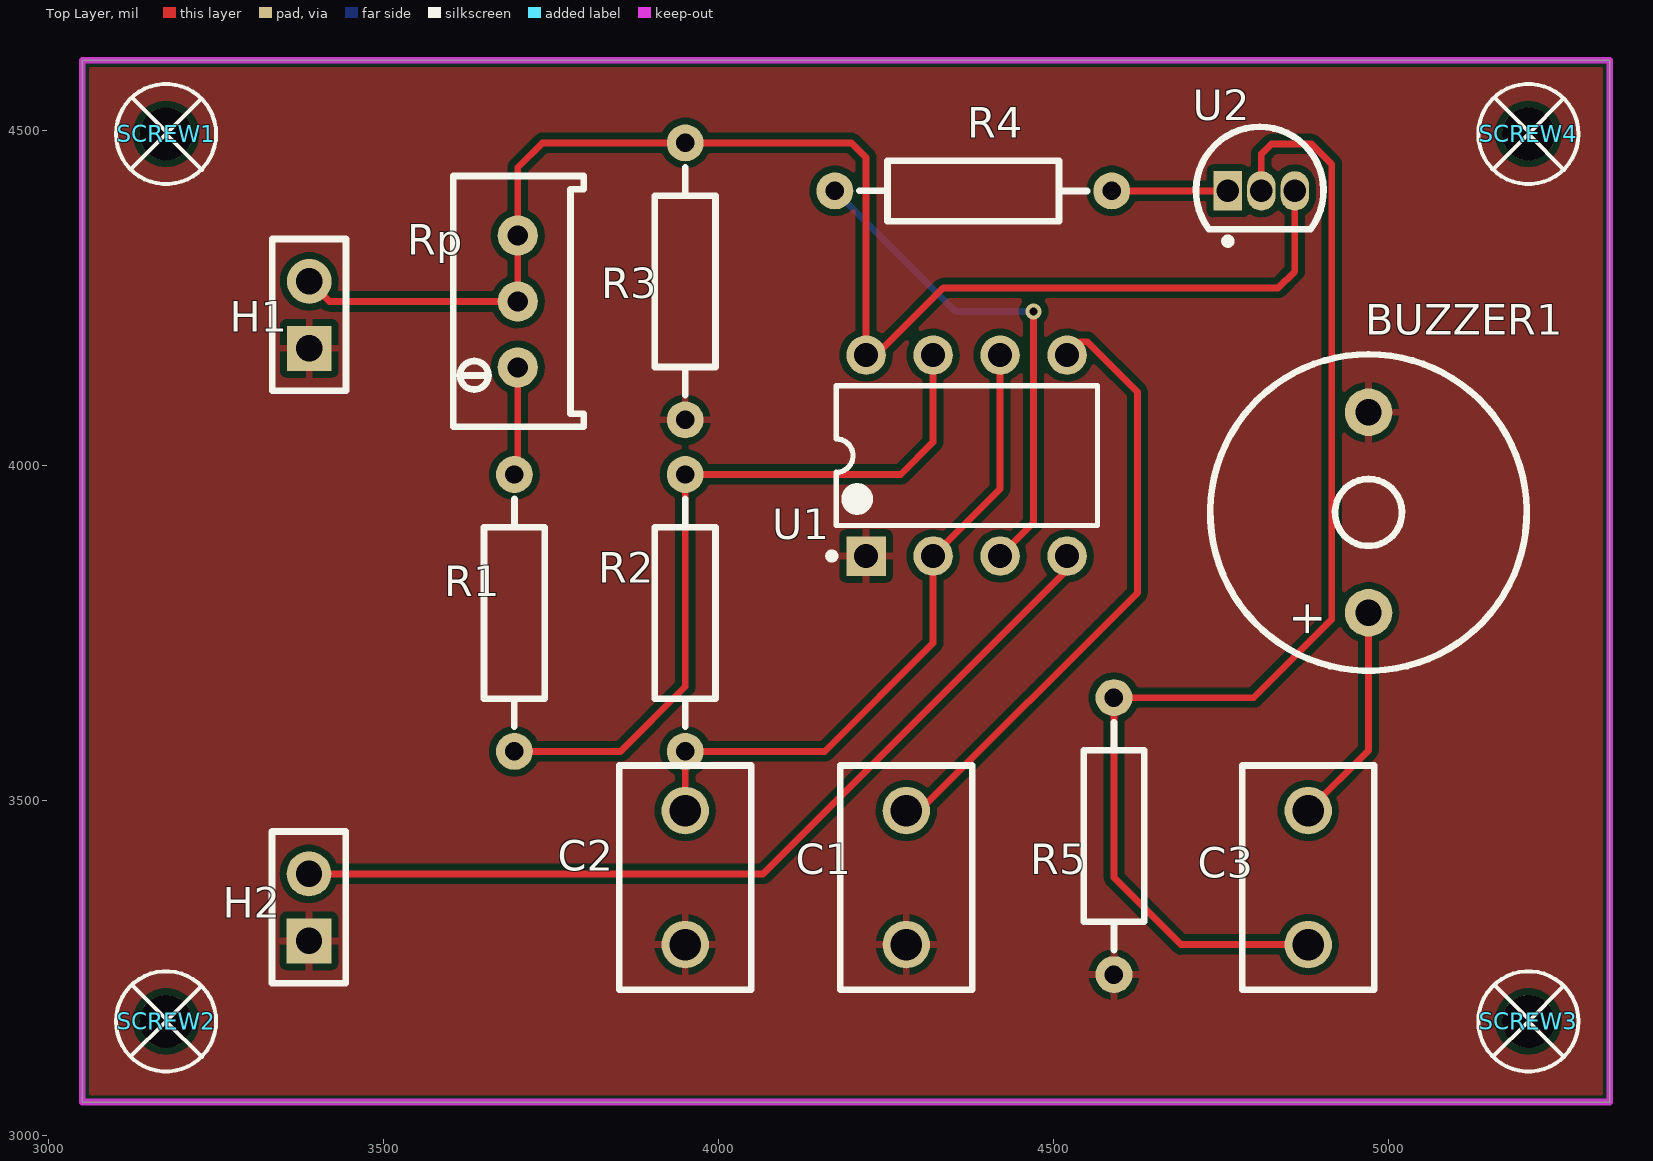
[diagram p0: Top Layer view]
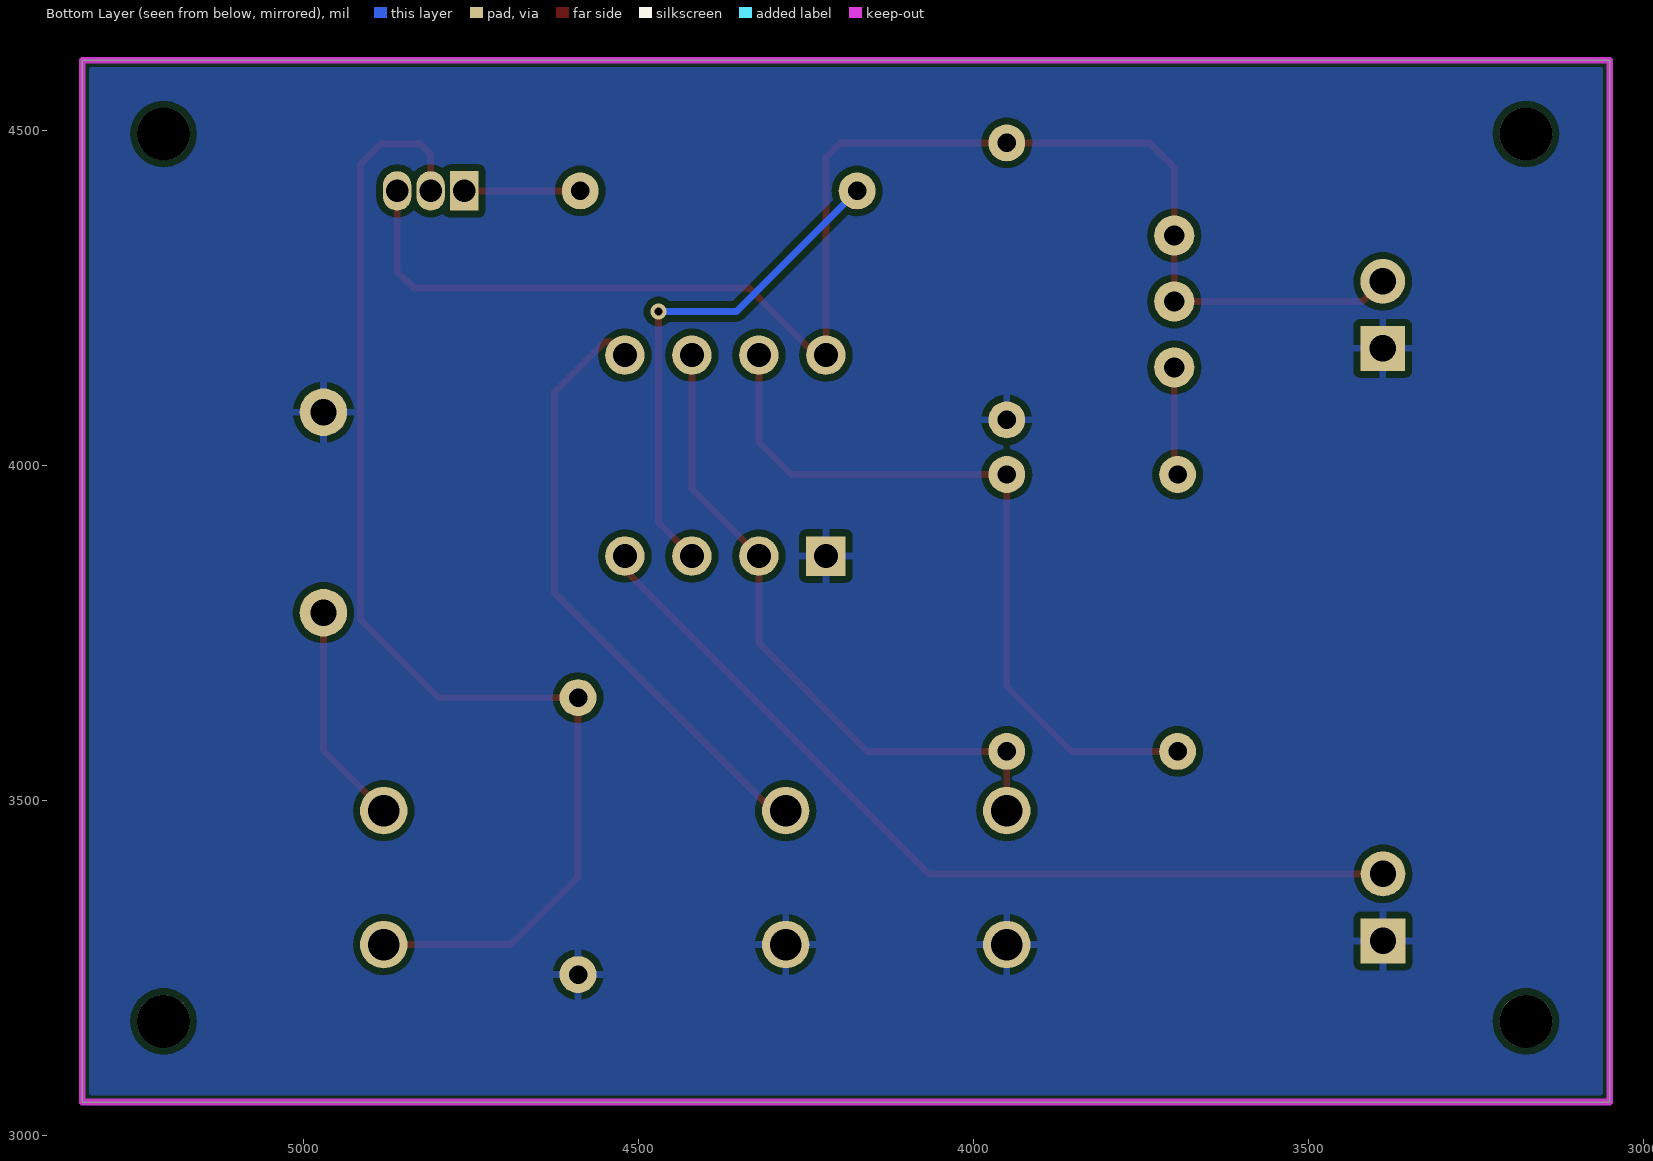
[diagram p1: Bottom Layer view, seen from below]
# Altium PCB MISC51754.pcbdoc
Units mil, origin at the board's own origin, x right, y up, seen from the top; angles counter-clockwise.
Board outline 2280 x 1555 mil, 2 copper layers (Top Layer, Bottom Layer), stack 62.206 mil thick; 18 components, 11 nets, 40 pads, 1 vias.

## Layer stack, top to bottom
Top Solder Mask Layer: solder mask 0.394, Dk 3.3
Top Layer: signal copper 1.379
Dielectric1: surface 59.449, FR4, Dk 4.5
Bottom Layer: signal copper 1.378
Bottom Solder Mask Layer: solder mask 0.394, Dk 3.3

## Board outline
3050,4605 3050,3050 5330,3050 5330,4605

## Design rules (kind name [scope] priority, off if disabled: settings)
BoardOutlineClearance copperThickness2oz_1 [All] p2 off: genericclearance=7.99 ignorepadtopadclearanceinfootprint=FALSE except(0: Arc-SplitContinuation Track-SplitContinuation SMDPad-SplitContinuation THPad-SplitContinuation Via-SplitContinuation Fill-SplitContinuation Region-SplitContinuation Poly-SplitContinuation Text-SplitContinuation Hole-SplitContinuation; 5.98: SMDPad-CutoutEdge THPad-CutoutEdge Via-CutoutEdge Fill-CutoutEdge Region-CutoutEdge Text-CutoutEdge Hole-CutoutEdge; 10: Poly-OutlineEdge Poly-CutoutEdge; 11.81: Arc-OutlineEdge Track-OutlineEdge SMDPad-OutlineEdge THPad-OutlineEdge Via-OutlineEdge Fill-OutlineEdge Region-OutlineEdge Text-OutlineEdge Hole-OutlineEdge Arc-CutoutEdge Track-CutoutEdge)
BoardOutlineClearance Plane_innerPlane_1 [All] p4 off: genericclearance=4.02 ignorepadtopadclearanceinfootprint=FALSE except(0: Arc-SplitContinuation Track-SplitContinuation SMDPad-SplitContinuation THPad-SplitContinuation Via-SplitContinuation Fill-SplitContinuation Region-SplitContinuation Poly-SplitContinuation Text-SplitContinuation Hole-SplitContinuation; 5.98: SMDPad-CutoutEdge THPad-CutoutEdge Via-CutoutEdge Fill-CutoutEdge Region-CutoutEdge Text-CutoutEdge Hole-CutoutEdge; 10: Poly-OutlineEdge Poly-CutoutEdge; 11.81: Arc-OutlineEdge Track-OutlineEdge SMDPad-OutlineEdge THPad-OutlineEdge Via-OutlineEdge Fill-OutlineEdge Region-OutlineEdge Text-OutlineEdge Hole-OutlineEdge Arc-CutoutEdge Track-CutoutEdge)
BoardOutlineClearance Copper_copperRegion_1 [All] p6 off: genericclearance=4.02 ignorepadtopadclearanceinfootprint=FALSE except(0: Arc-SplitContinuation Track-SplitContinuation SMDPad-SplitContinuation THPad-SplitContinuation Via-SplitContinuation Fill-SplitContinuation Region-SplitContinuation Poly-SplitContinuation Text-SplitContinuation Hole-SplitContinuation; 5.98: SMDPad-CutoutEdge THPad-CutoutEdge Via-CutoutEdge Fill-CutoutEdge Region-CutoutEdge Text-CutoutEdge Hole-CutoutEdge; 10: Poly-OutlineEdge Poly-CutoutEdge; 11.81: Arc-OutlineEdge Track-OutlineEdge SMDPad-OutlineEdge THPad-OutlineEdge Via-OutlineEdge Fill-OutlineEdge Region-OutlineEdge Text-OutlineEdge Hole-OutlineEdge Arc-CutoutEdge Track-CutoutEdge)
BoardOutlineClearance copperThickness1oz_1 [All] p8: genericclearance=4.02 ignorepadtopadclearanceinfootprint=FALSE except(0: Arc-SplitContinuation Track-SplitContinuation SMDPad-SplitContinuation THPad-SplitContinuation Via-SplitContinuation Fill-SplitContinuation Region-SplitContinuation Poly-SplitContinuation Text-SplitContinuation Hole-SplitContinuation; 5.98: SMDPad-CutoutEdge THPad-CutoutEdge Via-CutoutEdge Fill-CutoutEdge Region-CutoutEdge Text-CutoutEdge Hole-CutoutEdge; 10: Poly-OutlineEdge Poly-CutoutEdge; 11.81: Arc-OutlineEdge Track-OutlineEdge SMDPad-OutlineEdge THPad-OutlineEdge Via-OutlineEdge Fill-OutlineEdge Region-OutlineEdge Text-OutlineEdge Hole-OutlineEdge Arc-CutoutEdge Track-CutoutEdge)
Clearance copperThickness2oz [All] p1 off: gap=7.99 ignorepadtopadclearanceinfootprint=FALSE except(5.98: SMDPad-Track SMDPad-SMDPad THPad-Track SMDPad-THPad THPad-THPad Track-Via SMDPad-Via THPad-Via Via-Via Fill-Track Region-Track Fill-SMDPad Region-SMDPad Fill-THPad Region-THPad Fill-Via Region-Via Fill-Fill Fill-Region Region-Region Arc-Track Arc-SMDPad Arc-THPad Arc-Via Fill-Arc Region-Arc Arc-Arc Text-Track SMDPad-Text Text-THPad Text-Via Fill-Text Region-Text Arc-Text Text-Text Hole-Track Hole-SMDPad Hole-THPad Hole-Via Fill-Hole Region-Hole Hole-Arc Hole-Text; 10: Poly-Track Poly-SMDPad Poly-THPad Poly-Via Poly-Fill Poly-Region Poly-Poly Poly-Arc Poly-Text Poly-Hole)
Clearance Plane_innerPlane [All] p3 off: gap=4.02 ignorepadtopadclearanceinfootprint=FALSE except(5.98: SMDPad-Track SMDPad-SMDPad THPad-Track SMDPad-THPad THPad-THPad Track-Via SMDPad-Via THPad-Via Via-Via Fill-Track Region-Track Fill-SMDPad Region-SMDPad Fill-THPad Region-THPad Fill-Via Region-Via Fill-Fill Fill-Region Region-Region Arc-Track Arc-SMDPad Arc-THPad Arc-Via Fill-Arc Region-Arc Arc-Arc Text-Track SMDPad-Text Text-THPad Text-Via Fill-Text Region-Text Arc-Text Text-Text Hole-Track Hole-SMDPad Hole-THPad Hole-Via Fill-Hole Region-Hole Hole-Arc Hole-Text; 10: Poly-Track Poly-SMDPad Poly-THPad Poly-Via Poly-Fill Poly-Region Poly-Poly Poly-Arc Poly-Text Poly-Hole)
Clearance Copper_copperRegion [All] p5 off: gap=4.02 ignorepadtopadclearanceinfootprint=FALSE except(5.98: SMDPad-Track SMDPad-SMDPad THPad-Track SMDPad-THPad THPad-THPad Track-Via SMDPad-Via THPad-Via Via-Via Fill-Track Region-Track Fill-SMDPad Region-SMDPad Fill-THPad Region-THPad Fill-Via Region-Via Fill-Fill Fill-Region Region-Region Arc-Track Arc-SMDPad Arc-THPad Arc-Via Fill-Arc Region-Arc Arc-Arc Text-Track SMDPad-Text Text-THPad Text-Via Fill-Text Region-Text Arc-Text Text-Text Hole-Track Hole-SMDPad Hole-THPad Hole-Via Fill-Hole Region-Hole Hole-Arc Hole-Text; 10: Poly-Track Poly-SMDPad Poly-THPad Poly-Via Poly-Fill Poly-Region Poly-Poly Poly-Arc Poly-Text Poly-Hole)
Clearance copperThickness1oz [All] p7: gap=4.02 ignorepadtopadclearanceinfootprint=FALSE except(5.98: SMDPad-Track SMDPad-SMDPad THPad-Track SMDPad-THPad THPad-THPad Track-Via SMDPad-Via THPad-Via Via-Via Fill-Track Region-Track Fill-SMDPad Region-SMDPad Fill-THPad Region-THPad Fill-Via Region-Via Fill-Fill Fill-Region Region-Region Arc-Track Arc-SMDPad Arc-THPad Arc-Via Fill-Arc Region-Arc Arc-Arc Text-Track SMDPad-Text Text-THPad Text-Via Fill-Text Region-Text Arc-Text Text-Text Hole-Track Hole-SMDPad Hole-THPad Hole-Via Fill-Hole Region-Hole Hole-Arc Hole-Text; 10: Poly-Track Poly-SMDPad Poly-THPad Poly-Via Poly-Fill Poly-Region Poly-Poly Poly-Arc Poly-Text Poly-Hole)
DiffPairsRouting differentialPair [All] p1: maxlimit=6 minlimit=6 mostfreqgap=6 toplayer_minwidth=5 toplayer_prefwidth=10 toplayer_maxwidth=100 toplayer_mingap=6 toplayer_prefgap=6 toplayer_maxgap=6 bottomlayer_minwidth=5 bottomlayer_prefwidth=10 bottomlayer_maxwidth=100 bottomlayer_mingap=6 bottomlayer_prefgap=6 bottomlayer_maxgap=6 maxuncoupledlength=10
HoleToHoleClearance otherClearance [All] p1: gap=11.8 allowstackedmicrovias=TRUE
Length netLength [All] p1: minlimit=0 maxlimit=0
PasteMaskExpansion pasteMaskExpansion [All] p1: expansion=0
PlaneConnect innerPlane [All] p1: planeconnectstyle=Relief reliefexpansion=20 reliefentries=4 reliefconductorwidth=10 reliefairgap=10
PolygonConnect copperRegion [All] p1: connectstyle=Relief reliefconductorwidth=10 reliefentries=4 polygonreliefangle="90 Angle" airgapwidth=10 via.connectstyle=Relief via.reliefconductorwidth=10 via.reliefentries=4 via.polygonreliefangle="90 Angle" via.airgapwidth=10
RoutingVias viaSize [All] p1: holewidth=12.01 width=24.02 viastyle="Through Hole" minholewidth=11.81 minwidth=19.68 maxholewidth=248.03 maxwidth=393.7
SolderMaskExpansion solderMaskExpansion [IsVia] p1: expansion=-1000 istentingtop=TRUE
SolderMaskExpansion solderMaskExpansion [All] p2: expansion=2 istentingtop=FALSE
Width copperThickness2oz_2 [All] p1 off: maxlimit=100 minlimit=8 preferedwidth=10
Width copperThickness1oz_2 [All] p2: maxlimit=100 minlimit=5 preferedwidth=10

## Components (designator, comment, footprint, x,y, rotation, side; value= is the part's Value field where it differs from the comment)
BUZZER1 "" BUZ-TH_BD12.0-P7.60-D0.6-FD 4970,3930 r90 top
C1 "0.1uF" CAP-TH_L8.5-W5.0-P5.00-D1.2 4280,3385 r270 top
C2 "0.1uF" CAP-TH_L8.5-W5.0-P5.00-D1.2 3950,3385 r90 top
C3 "100uF" CAP-TH_L8.5-W5.0-P5.00-D1.2 4880,3385 r270 top
H1 "" HDR-TH_2P-P2.54-V-F 3388.79,4225 r90 top
H2 "" HDR-TH_2P-P2.54-V-F 3388.39,3340.49 r90 top
R1 "4.7kΩ" RES-TH_BD2.3-L6.5-P10.50-D0.5 3695,3780 r90 top
R2 "4.7kΩ" RES-TH_BD2.3-L6.5-P10.50-D0.5 3950,3780 r90 top
R3 "4.7kΩ" RES-TH_BD2.3-L6.5-P10.50-D0.5 3950,4275 r90 top
R4 "4.7kΩ" RES-TH_BD2.3-L6.5-P10.50-D0.5 4380,4410 r180 top
R5 "5.1kΩ" RES-TH_BD2.3-L6.5-P10.50-D0.5 4590,3446.93 r90 top
Rp "2kΩ" RES-ADJ-TH_3P-L10.0-W10.0-P2.50-BL-BS 3700,4245 r180 top
SCREW1 "" M2螺丝 3175,4495 r0 top
SCREW2 "" M2螺丝 3175,3170.35 r0 top
SCREW3 "" M2螺丝 5208.65,3170.35 r0 top
SCREW4 "" M2螺丝 5208.65,4495 r0 top
U1 "100kHz" DIP-8_L9.8-W6.6-P2.54-LS7.6-BL 4370,4015 r0 top
U2 "S9018" TO-92-3_L4.8-W3.7-P1.27-L 4810,4410 r0 top

## Footprints (in the part's own frame and the unit in brackets; to place one, negate y for a bottom-side part, rotate by r counter-clockwise, add the part's x,y. Pads: shape width x height; smd on the part's side, far side on the other; paste and mask are expansions set on the pad)
BUZ-TH_BD12.0-P7.60-D0.6-FD [mm]
  round 1.8 hole 1: 1(-3.8,0) 2(3.8,0)
  silkscreen extent -6,-6 6,6
CAP-TH_L8.5-W5.0-P5.00-D1.2 [mm]
  round 1.8 hole 1.2: 1(-2.54,0) 2(2.54,0)
  silkscreen extent -4.25,-2.5 4.25,2.5
DIP-8_L9.8-W6.6-P2.54-LS7.6-BL [mm]
  rect 1.5x1.5 hole 0.9: 1(-3.81,-3.81)
  round 1.5 hole 0.9: 2(-1.27,-3.81) 3(1.27,-3.81) 4(3.81,-3.81) 5(3.81,3.81) 6(1.27,3.81) 7(-1.27,3.81) 8(-3.81,3.81)
  silkscreen extent -5.23,-3.93 4.96,2.65
HDR-TH_2P-P2.54-V-F [mm]
  rect 1.7x1.7 hole 1: 1(-1.27,0)
  round 1.7 hole 1: 2(1.27,0)
  silkscreen extent -2.88,-1.39 2.88,1.4
M2螺丝 [mm]
  round 2 hole 2: 1(0,0)
  silkscreen extent -1.9,-1.9 1.9,1.9
RES-ADJ-TH_3P-L10.0-W10.0-P2.50-BL-BS [mil]
  round 60 hole 30: 1(0,98.43) 2(0.01,-0.01) 3(0,-98.43)
  silkscreen extent -98,-187 96,187
RES-TH_BD2.3-L6.5-P10.50-D0.5 [mm]
  round 1.4 hole 0.7: 1(-5.25,0) 2(5.25,0)
  silkscreen extent -4.32,-1.15 4.32,1.15
TO-92-3_L4.8-W3.7-P1.27-L [mm]
  rect 1.07x1.5 hole 0.85: 1(-1.27,0)
  oval 1.07x1.5 hole 0.85: 2(0,0) 3(1.27,0)
  silkscreen extent -2.48,-2.03 2.36,2.43

## Via types
v1: diameter 24.02, hole 12, Top Layer to Bottom Layer, 1 vias

## Nets (pads, with @x,y where several pads share a name; then routed paths per layer and width w, separated by ;. In a path a pad name is that pad's centre, name@x,y a point inside that pad or via, vN(x,y) a via of type N, cw(c..) or ccw(c..) an arc to the next point about the centre after c; other vN are vias at no path point)
$1N476: C1.1 U1.5 | length 924
  Top Layer w10: C1.1 4300,3485 4625,3810 4625,4110 4550,4185 4540,4185 U1.5
$1N1069: R1.2 Rp.1 | length 162
  Top Layer w10: R1.2 3700,3991.69 Rp.1
$1N1211: R1.1 R2.2 U1.7 | length 1131.8
  Top Layer w10: R1.1 3853.31,3573.31 3950,3670 R2.2 4271.69,3986.69 4320,4035 U1.7
$1N1246: C2.2 R2.1 U1.2 U1.6 | length 996.7
  Top Layer w10: C2.2 R2.1 4158.31,3573.31 4320,3735 U1.2 4420,3965 U1.6
$1N1349: R4.1 U2.1 | length 166.5
  Top Layer w10: R4.1 U2.1@4753.23,4410
$1N1352: H1.2 R3.2 Rp.2 Rp.3 U1.8 U2.3 | length 2174.6
  Top Layer w10: H1.2 3418.78,4245.01 Rp.2 Rp.3 3700,4445 3736.69,4481.69 R3.2 4198.31,4481.69 4220,4460 U1.8 4235,4165 4335,4265 4835,4265 4860,4290 U2.3
$1N1384: C3.2 R5.2 U2.2 | length 1831.9
  Top Layer w10: U2.2 4810,4465 4825,4480 4885,4480 4915,4450 4915,3770 4798.61,3653.61 R5.2 4590,3385 4690,3285 C3.2
$1N1510: R4.2 U1.3 | length 757
  Top Layer w10: U1.3 4470,3915 v1(4470,4230)
  Bottom Layer w10: R4.2 4353.31,4230 v1(4470,4230)
$1N1645: BUZZER1.1 C3.1 | length 332.7
  Top Layer w10: C3.1 4970,3575 BUZZER1.1
$1N1944: H2.2 U1.4 | length 1340.3
  Top Layer w10: H2.2 4066.21,3390.49 4520,3844.29 U1.4
GND: BUZZER1.2 C1.2 C2.1 H1.1 H2.1 R3.1 R5.1 U1.1
pads on no net: SCREW1.1 SCREW2.1 SCREW3.1 SCREW4.1

## Polygon pours and split planes (outlines as drawn)
GND on Top Layer (solid, remove dead copper, pour order 0): 3010,4655 3010,3000 5385,3000 5385,4655
GND on Bottom Layer (solid, remove dead copper, pour order 2): 3000,4640 3000,3000 5385,3000 5385,4640

## Keep-outs
Board Outline Layer:
  the board outline again, w10